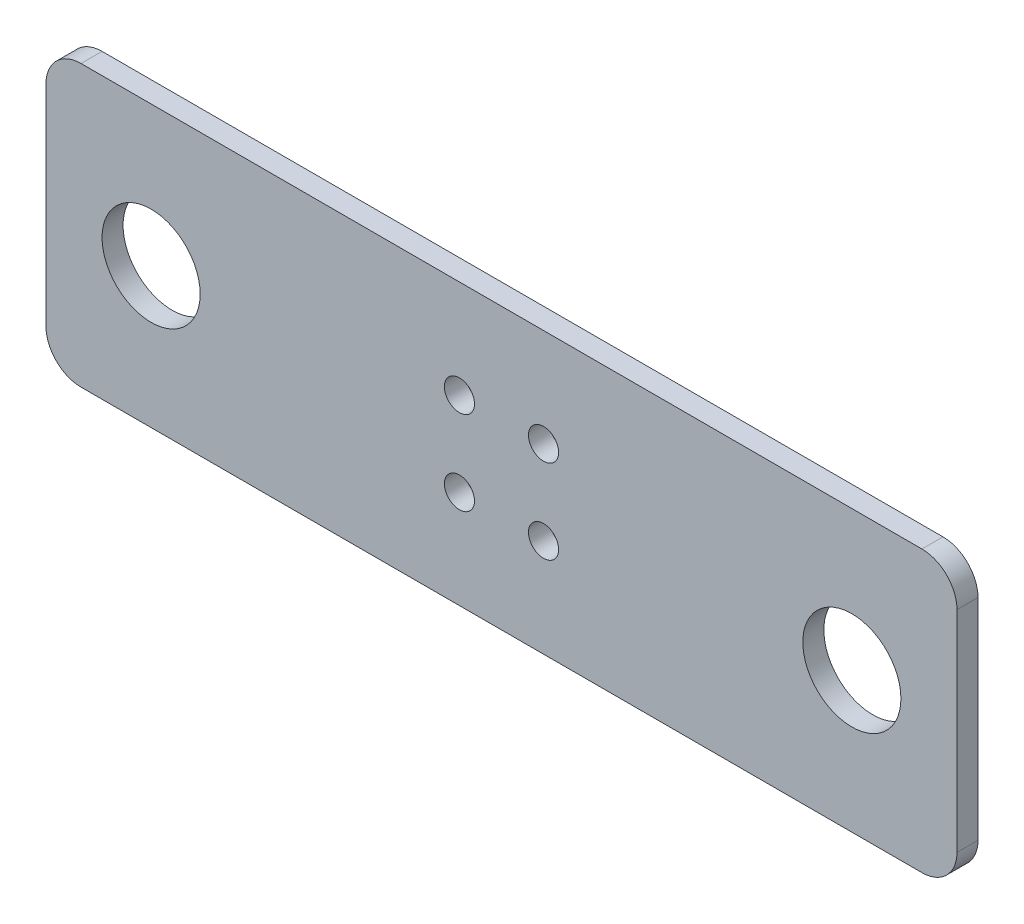
from build123d import *

# Parameters (mm, degrees)
SKETCH_1_W          = 130
SKETCH_1_H          = 40
EXTRUDE_1_DEPTH     = 3
SKETCH_2_R          = 7
SKETCH_2_R_2        = 2.15
CUT_EXTRUDE_1_DEPTH = 3
FILLET_1_R          = 5


with BuildPart() as part:
    # 草图1 → 凸台-拉伸1 (new body)
    with BuildSketch(Plane.XY):
        Rectangle(SKETCH_1_W, SKETCH_1_H)
    extrude(amount=EXTRUDE_1_DEPTH)

    # 草图2 → 切除-拉伸1 (cut)
    with BuildSketch(Plane.XY.offset(3)):
        with Locations((-50, 0)):
            Circle(SKETCH_2_R)
        with Locations((50, 0)):
            Circle(SKETCH_2_R)
        with Locations((-6, 6)):
            Circle(SKETCH_2_R_2)
        with Locations((6, 6)):
            Circle(SKETCH_2_R_2)
        with Locations((6, -6)):
            Circle(SKETCH_2_R_2)
        with Locations((-6, -6)):
            Circle(SKETCH_2_R_2)
    extrude(amount=-CUT_EXTRUDE_1_DEPTH, mode=Mode.SUBTRACT)

    # 圆角1
    fillet_1_edges = [part.edges().sort_by_distance(p)[0] for p in [
        (65, -20, 1.5),
        (-65, -20, 1.5),
        (-65, 20, 1.5),
        (65, 20, 1.5),
    ]]
    fillet(fillet_1_edges, radius=FILLET_1_R)


solid = part.part
